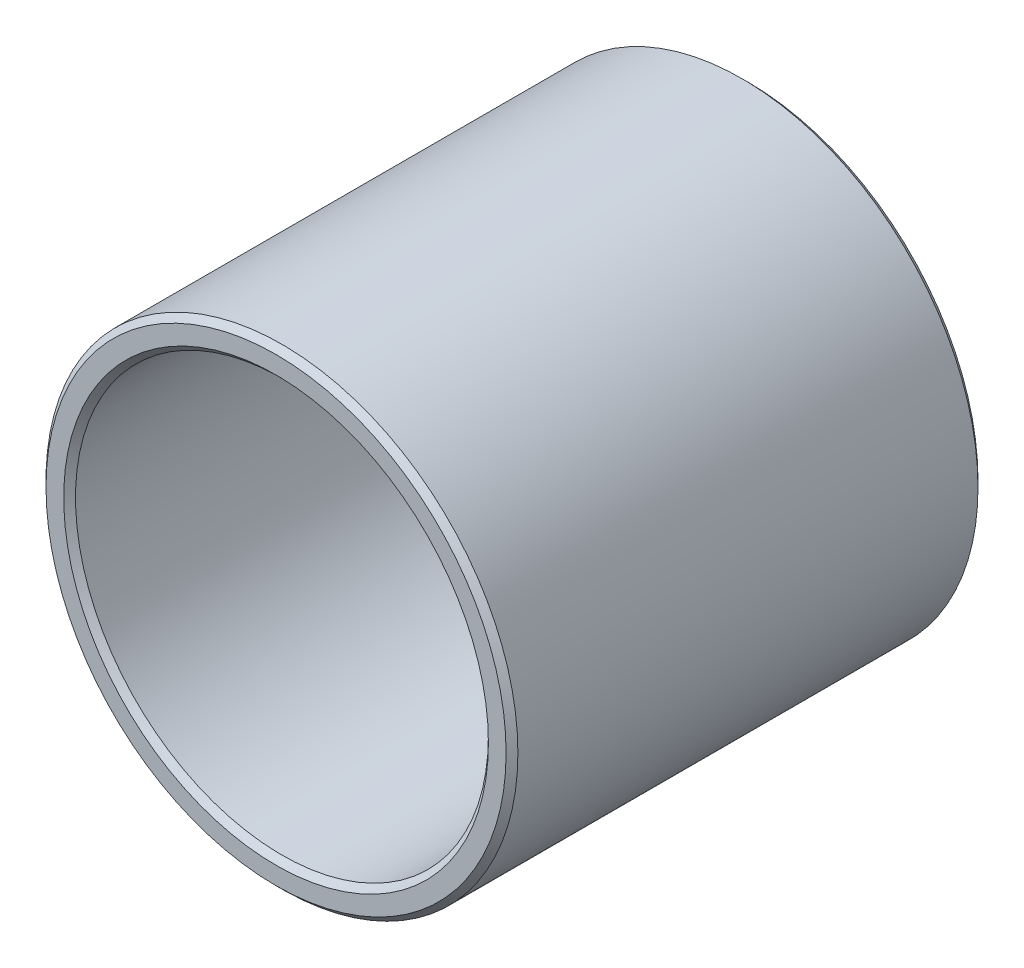
SolidWorks part; units mm, degrees
material "ZCuSn10Pb5"
ref_plane "Front Plane" through (0, 0, 0) normal (0, 0, 1) x (1, 0, 0)
ref_plane "Top Plane" through (0, 0, 0) normal (0, 1, 0) x (1, 0, 0)
ref_plane "Right Plane" through (0, 0, 0) normal (1, 0, 0) x (0, 0, -1)
sketch "Sketch1" plane through (0, 0, 0) normal (0, 0, 1) x (1, 0, 0)
  circle A0 centre (0, 0) radius 35
  circle A1 centre (0, 0) radius 40
  dimension "D1" = 70
  dimension "D2" = 80
extrude "Boss-Extrude1" add sketch "Sketch1" along normal mid plane 80
chamfer "Chamfer1" distance 1 angle 45 4 edges at (40, 0, -40) (35, 0, -40) (40, 0, 40) (35, 0, 40)
